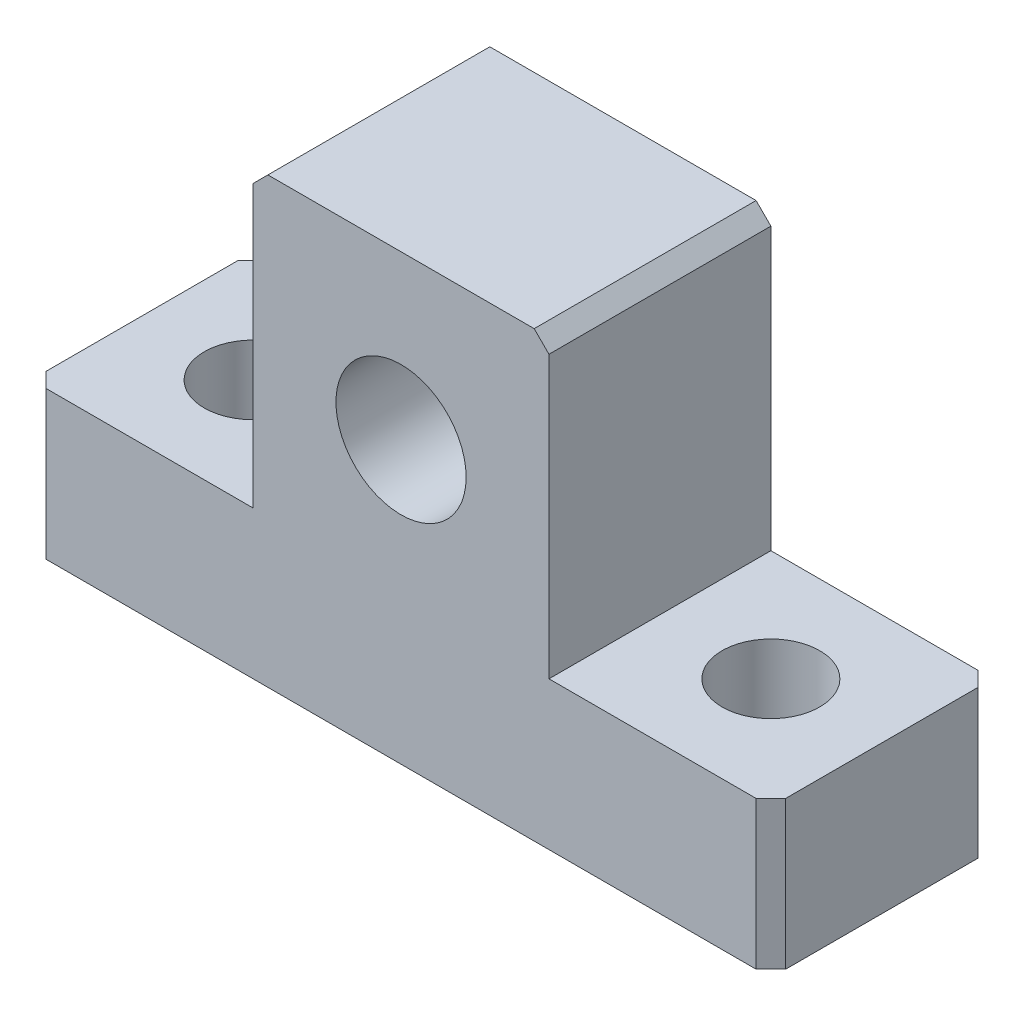
SolidWorks part; units mm, degrees
material "Q235-A"
ref_plane "Front Plane" through (0, 0, 0) normal (0, 0, 1) x (1, 0, 0)
ref_plane "Top Plane" through (0, 0, 0) normal (0, 1, 0) x (1, 0, 0)
ref_plane "Right Plane" through (0, 0, 0) normal (1, 0, 0) x (0, 0, -1)
sketch "Sketch1" plane through (0, 0, 0) normal (0, 0, 1) x (1, 0, 0)
  line L0 (-7.9216, 21.7219) -> (-7.9216, 1.7219)
  line L1 (-7.9216, 1.7219) -> (-22.9216, 1.7219)
  line L2 (-22.9216, 1.7219) -> (-22.9216, -8.2781)
  line L3 (-22.9216, -8.2781) -> (27.0784, -8.2781)
  line L4 (27.0784, -8.2781) -> (27.0784, 1.7219)
  line L5 (27.0784, 1.7219) -> (12.0784, 1.7219)
  line L6 (12.0784, 1.7219) -> (12.0784, 21.7219)
  line L7 (12.0784, 21.7219) -> (-7.9216, 21.7219)
  dimension "D1" = 50
  dimension "D2" = 30
  dimension "D3" = 10
  dimension "D4" = 10
  dimension "D5" = 20
  dimension "D6" = 15
extrude "Boss-Extrude1" add sketch "Sketch1" along normal blind 15
chamfer "Chamfer1" distance 1 angle 45 6 edges at (27.0784, -3.2781, 15) (27.0784, -3.2781, 0) (-22.9216, -3.2781, 15) (-22.9216, -3.2781, 0) (12.0784, 21.7219, 7.5) (-7.9216, 21.7219, 7.5)
sketch "Sketch2" plane through (0, 1.7219, 0) normal (0, 1, 0) x (1, 0, 0)
  line L0 (-15.4216, -7.5) -> (19.5784, -7.5)
  line L1 (27.0784, -14) -> (27.0784, -1) construction
  dimension "D1" = 35
  dimension "D2" = 7.5
hole_wizard "Hole1" positions "Sketch3" profile "Sketch4" legacy end condition through all
sketch "Sketch3" plane through (0, 1.7219, 0) normal (0, 1, 0) x (1, 0, 0)
  point P0 (-15.4216, -7.5)
  point P3 (19.5784, -7.5)
sketch "Sketch4" plane through (-15.4216, 1.7219, 7.5) normal (1, 0, 0) x (0, 0, 1)
  line L0 (0, 0) -> (0, 10)
  line L1 (0, 10) -> (3.3, 10)
  line L2 (3.3, 10) -> (3.3, 0)
  line L3 (3.3, 0) -> (0, 0)
  line L4 (0, 110) -> (0, -10) construction
  dimension "直径" = 6.6
  dimension "深度" = 10
sketch "Sketch5" plane through (0, 0, 15) normal (0, 0, 1) x (1, 0, 0)
  line L0 (-21.9216, -8.2781) -> (26.0784, -8.2781) construction
  circle A0 centre (2.0784, 10.7219) radius 2.5144
  dimension "D1" = 19
hole_wizard "M10x1.25 Tapped Hole1" positions "Sketch6" profile "Sketch7" tap size "M10x1.25" standard "GB" end condition through all
sketch "Sketch6" plane through (0, 0, 15) normal (0, 0, 1) x (1, 0, 0)
  point P0 (2.0784, 10.7219)
sketch "Sketch7" plane through (2.0784, 10.7219, 15) normal (1, 0, 0) x (0, -1, 0)
  line L0 (0, 0) -> (0, 15)
  line L1 (0, 15) -> (4.4, 15)
  line L2 (4.4, 15) -> (4.4, 0)
  line L5 (4.4, 0) -> (0, 0)
  line L11 (0, -6.35) -> (0, 107.95) construction
  dimension "通孔螺纹孔钻头直径" = 8.8
  dimension "通孔螺纹孔钻头深度" = 15
cosmetic thread "Cosmetic thread 1" parameters "D2"=10
